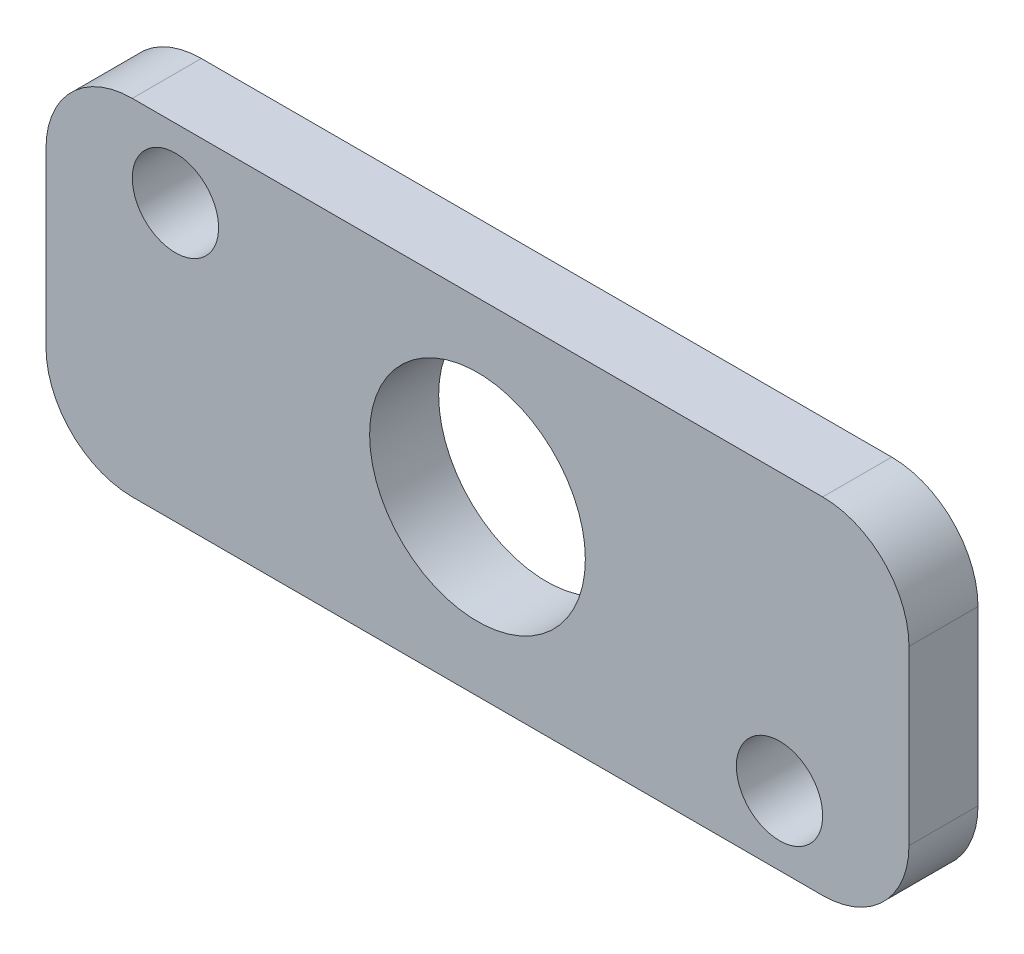
from build123d import *

# Parameters (mm, degrees)
SKETCH_1_R      = 2.5
SKETCH_1_R_2    = 6.25
EXTRUDE_1_DEPTH = 4


with BuildPart() as part:
    # 草图1 → 凸台-拉伸1 (new body)
    with BuildSketch(Plane.XY.offset(2)):
        with BuildLine():
            Line((-20, -10), (20, -10))
            ThreePointArc((20, -10), (23.535533906, -8.535533906), (25, -5))
            Line((25, -5), (25, 5))
            ThreePointArc((25, 5), (23.535533906, 8.535533906), (20, 10))
            Line((20, 10), (-20, 10))
            ThreePointArc((-20, 10), (-23.535533906, 8.535533906), (-25, 5))
            Line((-25, 5), (-25, -5))
            ThreePointArc((-25, -5), (-23.535533906, -8.535533906), (-20, -10))
        make_face()
        with Locations(Location((-17.5, 6, 0), (0, 0, 180))):
            Circle(SKETCH_1_R, mode=Mode.SUBTRACT)
        with Locations(Location((17.5, -6, 0), (0, 0, 180))):
            Circle(SKETCH_1_R, mode=Mode.SUBTRACT)
        with Locations(Location((0, 0, 0), (0, 0, 180))):
            Circle(SKETCH_1_R_2, mode=Mode.SUBTRACT)
    extrude(amount=-EXTRUDE_1_DEPTH)


solid = part.part
